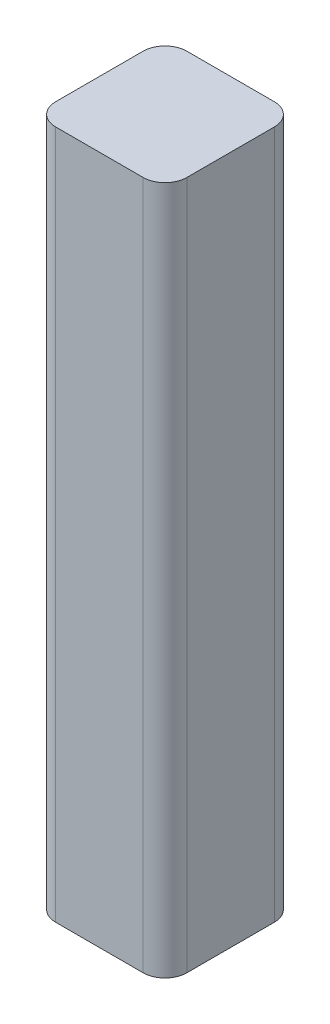
SolidWorks part; units mm, degrees
ref_plane "Front Plane" through (0, 0, 0) normal (0, 0, 1) x (1, 0, 0)
ref_plane "Top Plane" through (0, 0, 0) normal (0, 1, 0) x (1, 0, 0)
ref_plane "Right Plane" through (0, 0, 0) normal (1, 0, 0) x (0, 0, -1)
ref_plane "Plane4" through (0, 0, 0) normal (0, -1, 0) x (1, 0, 0)
sketch "Sketch1" plane through (0, 0, 0) normal (0, -1, 0) x (1, 0, 0)
  line L0 (40, -26.6667) -> (40, 26.6667)
  line L1 (26.6667, 40) -> (-26.6667, 40)
  line L2 (-40, 26.6667) -> (-40, -26.6667)
  line L3 (-26.6667, -40) -> (26.6667, -40)
  arc A0 (40, 26.6667) -> (26.6667, 40) centre (26.6667, 26.6667) ccw
  arc A1 (-26.6667, 40) -> (-40, 26.6667) centre (-26.6667, 26.6667) ccw
  arc A2 (-40, -26.6667) -> (-26.6667, -40) centre (-26.6667, -26.6667) ccw
  arc A3 (26.6667, -40) -> (40, -26.6667) centre (26.6667, -26.6667) ccw
  dimension "D1" = 80
extrude "Boss-Extrude1" add sketch "Sketch1" against normal blind 420
